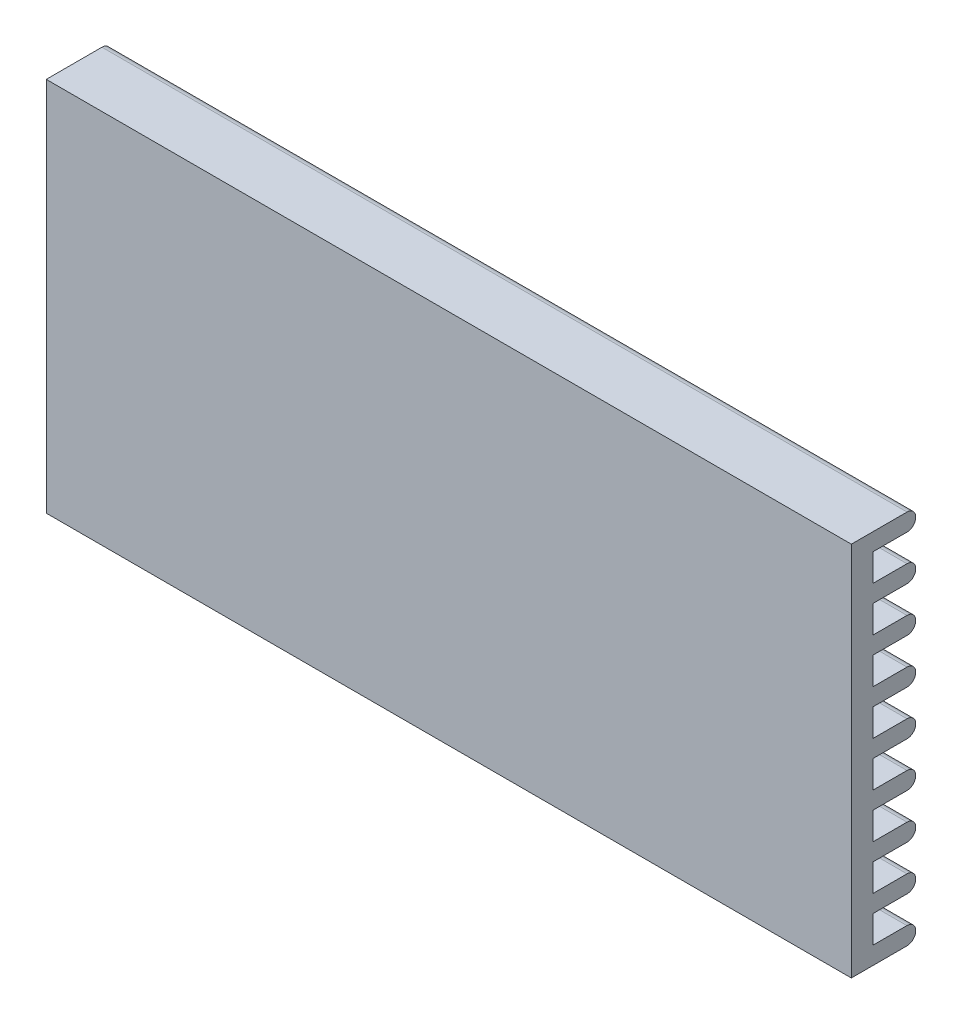
from build123d import *

# Parameters (mm, degrees)
SKETCH_1_W             = 75
SKETCH_1_H             = 35
EXTRUDE_1_DEPTH        = 6
SKETCH_2_W             = 75
SKETCH_2_H             = 2.55
CUT_EXTRUDE_1_DEPTH    = 4
PATTERN_LINEAR_1_COUNT = 8
PATTERN_LINEAR_1_PITCH = 4.17
FILLET_2_RADIUS        = 0.81
FILLET_2_LENGTH        = 75
FILLET_3_RADIUS        = 0.81
FILLET_3_LENGTH        = 75
FILLET_4_RADIUS        = 0.81
FILLET_4_LENGTH        = 75
FILLET_5_RADIUS        = 0.81
FILLET_5_LENGTH        = 75
FILLET_6_RADIUS        = 0.81
FILLET_6_LENGTH        = 75
FILLET_7_RADIUS        = 0.81
FILLET_7_LENGTH        = 75
FILLET_8_RADIUS        = 0.81
FILLET_8_LENGTH        = 75
FILLET_9_RADIUS        = 0.81
FILLET_9_LENGTH        = 75
FILLET_10_RADIUS       = 0.82
FILLET_10_LENGTH       = 75


with BuildPart() as part:
    # 草图1 → 拉伸1 (new body)
    with BuildSketch(Plane.XY):
        Rectangle(SKETCH_1_W, SKETCH_1_H)
    extrude(amount=EXTRUDE_1_DEPTH)

    # 草图2 → 切除-拉伸1 (cut)
    with BuildSketch(Plane(origin=(0, 0, 0), x_dir=(-1, 0, 0), z_dir=(0, 0, -1))):
        with Locations((0, 14.605)):
            Rectangle(SKETCH_2_W, SKETCH_2_H)
    cut_extrude_1 = extrude(amount=-CUT_EXTRUDE_1_DEPTH, mode=Mode.SUBTRACT)

    # 阵列(线性)1: 切除-拉伸1 ×8
    with Locations(*[(0, -i * PATTERN_LINEAR_1_PITCH, 0) for i in range(1, PATTERN_LINEAR_1_COUNT)]):
        add(cut_extrude_1, mode=Mode.SUBTRACT)

    # 圆角2: full round fillet: the end face becomes a half cylinder, R = half its width
    fillet_2_face = Plane((0, 16.69, 0), x_dir=(-1, 0, 0), z_dir=(0, 0, -1))  # on the end face: x along it, z out of the body
    fillet_2_slab = fillet_2_face.offset(-FILLET_2_RADIUS / 2) * Box(FILLET_2_LENGTH, 2 * FILLET_2_RADIUS, FILLET_2_RADIUS, mode=Mode.PRIVATE)  # the body's end, R deep
    fillet_2_round = Plane((0, 16.69, 0.81), x_dir=(0, 0, -1), z_dir=(-1, 0, 0)) * Cylinder(FILLET_2_RADIUS, FILLET_2_LENGTH, mode=Mode.PRIVATE)  # its axis R under the face
    add(fillet_2_slab - fillet_2_round, mode=Mode.SUBTRACT)

    # 圆角3: full round fillet: the end face becomes a half cylinder, R = half its width
    fillet_3_face = Plane((0, 12.52, 0), x_dir=(1, 0, 0), z_dir=(0, 0, -1))  # on the end face: x along it, z out of the body
    fillet_3_slab = fillet_3_face.offset(-FILLET_3_RADIUS / 2) * Box(FILLET_3_LENGTH, 2 * FILLET_3_RADIUS, FILLET_3_RADIUS, mode=Mode.PRIVATE)  # the body's end, R deep
    fillet_3_round = Plane((0, 12.52, 0.81), x_dir=(0, 0, -1), z_dir=(1, 0, 0)) * Cylinder(FILLET_3_RADIUS, FILLET_3_LENGTH, mode=Mode.PRIVATE)  # its axis R under the face
    add(fillet_3_slab - fillet_3_round, mode=Mode.SUBTRACT)

    # 圆角4: full round fillet: the end face becomes a half cylinder, R = half its width
    fillet_4_face = Plane((0, 8.35, 0), x_dir=(1, 0, 0), z_dir=(0, 0, -1))  # on the end face: x along it, z out of the body
    fillet_4_slab = fillet_4_face.offset(-FILLET_4_RADIUS / 2) * Box(FILLET_4_LENGTH, 2 * FILLET_4_RADIUS, FILLET_4_RADIUS, mode=Mode.PRIVATE)  # the body's end, R deep
    fillet_4_round = Plane((0, 8.35, 0.81), x_dir=(0, 0, -1), z_dir=(1, 0, 0)) * Cylinder(FILLET_4_RADIUS, FILLET_4_LENGTH, mode=Mode.PRIVATE)  # its axis R under the face
    add(fillet_4_slab - fillet_4_round, mode=Mode.SUBTRACT)

    # 圆角5: full round fillet: the end face becomes a half cylinder, R = half its width
    fillet_5_face = Plane((0, 4.18, 0), x_dir=(1, 0, 0), z_dir=(0, 0, -1))  # on the end face: x along it, z out of the body
    fillet_5_slab = fillet_5_face.offset(-FILLET_5_RADIUS / 2) * Box(FILLET_5_LENGTH, 2 * FILLET_5_RADIUS, FILLET_5_RADIUS, mode=Mode.PRIVATE)  # the body's end, R deep
    fillet_5_round = Plane((0, 4.18, 0.81), x_dir=(0, 0, -1), z_dir=(1, 0, 0)) * Cylinder(FILLET_5_RADIUS, FILLET_5_LENGTH, mode=Mode.PRIVATE)  # its axis R under the face
    add(fillet_5_slab - fillet_5_round, mode=Mode.SUBTRACT)

    # 圆角6: full round fillet: the end face becomes a half cylinder, R = half its width
    fillet_6_face = Plane((0, 0.01, 0), x_dir=(1, 0, 0), z_dir=(0, 0, -1))  # on the end face: x along it, z out of the body
    fillet_6_slab = fillet_6_face.offset(-FILLET_6_RADIUS / 2) * Box(FILLET_6_LENGTH, 2 * FILLET_6_RADIUS, FILLET_6_RADIUS, mode=Mode.PRIVATE)  # the body's end, R deep
    fillet_6_round = Plane((0, 0.01, 0.81), x_dir=(0, 0, -1), z_dir=(1, 0, 0)) * Cylinder(FILLET_6_RADIUS, FILLET_6_LENGTH, mode=Mode.PRIVATE)  # its axis R under the face
    add(fillet_6_slab - fillet_6_round, mode=Mode.SUBTRACT)

    # 圆角7: full round fillet: the end face becomes a half cylinder, R = half its width
    fillet_7_face = Plane((0, -4.16, 0), x_dir=(1, 0, 0), z_dir=(0, 0, -1))  # on the end face: x along it, z out of the body
    fillet_7_slab = fillet_7_face.offset(-FILLET_7_RADIUS / 2) * Box(FILLET_7_LENGTH, 2 * FILLET_7_RADIUS, FILLET_7_RADIUS, mode=Mode.PRIVATE)  # the body's end, R deep
    fillet_7_round = Plane((0, -4.16, 0.81), x_dir=(0, 0, -1), z_dir=(1, 0, 0)) * Cylinder(FILLET_7_RADIUS, FILLET_7_LENGTH, mode=Mode.PRIVATE)  # its axis R under the face
    add(fillet_7_slab - fillet_7_round, mode=Mode.SUBTRACT)

    # 圆角8: full round fillet: the end face becomes a half cylinder, R = half its width
    fillet_8_face = Plane((0, -8.33, 0), x_dir=(-1, 0, 0), z_dir=(0, 0, -1))  # on the end face: x along it, z out of the body
    fillet_8_slab = fillet_8_face.offset(-FILLET_8_RADIUS / 2) * Box(FILLET_8_LENGTH, 2 * FILLET_8_RADIUS, FILLET_8_RADIUS, mode=Mode.PRIVATE)  # the body's end, R deep
    fillet_8_round = Plane((0, -8.33, 0.81), x_dir=(0, 0, -1), z_dir=(-1, 0, 0)) * Cylinder(FILLET_8_RADIUS, FILLET_8_LENGTH, mode=Mode.PRIVATE)  # its axis R under the face
    add(fillet_8_slab - fillet_8_round, mode=Mode.SUBTRACT)

    # 圆角9: full round fillet: the end face becomes a half cylinder, R = half its width
    fillet_9_face = Plane((0, -12.5, 0), x_dir=(1, 0, 0), z_dir=(0, 0, -1))  # on the end face: x along it, z out of the body
    fillet_9_slab = fillet_9_face.offset(-FILLET_9_RADIUS / 2) * Box(FILLET_9_LENGTH, 2 * FILLET_9_RADIUS, FILLET_9_RADIUS, mode=Mode.PRIVATE)  # the body's end, R deep
    fillet_9_round = Plane((0, -12.5, 0.81), x_dir=(0, 0, -1), z_dir=(1, 0, 0)) * Cylinder(FILLET_9_RADIUS, FILLET_9_LENGTH, mode=Mode.PRIVATE)  # its axis R under the face
    add(fillet_9_slab - fillet_9_round, mode=Mode.SUBTRACT)

    # 圆角10: full round fillet: the end face becomes a half cylinder, R = half its width
    fillet_10_face = Plane((0, -16.68, 0), x_dir=(1, 0, 0), z_dir=(0, 0, -1))  # on the end face: x along it, z out of the body
    fillet_10_slab = fillet_10_face.offset(-FILLET_10_RADIUS / 2) * Box(FILLET_10_LENGTH, 2 * FILLET_10_RADIUS, FILLET_10_RADIUS, mode=Mode.PRIVATE)  # the body's end, R deep
    fillet_10_round = Plane((0, -16.68, 0.82), x_dir=(0, 0, -1), z_dir=(1, 0, 0)) * Cylinder(FILLET_10_RADIUS, FILLET_10_LENGTH, mode=Mode.PRIVATE)  # its axis R under the face
    add(fillet_10_slab - fillet_10_round, mode=Mode.SUBTRACT)


solid = part.part
